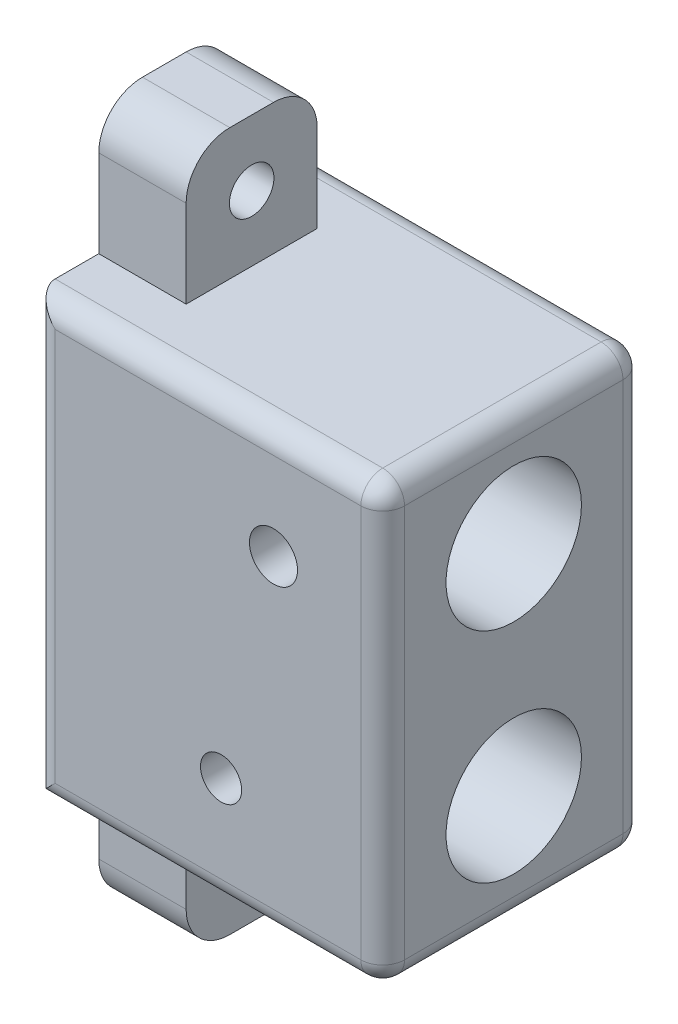
SolidWorks part; units mm, degrees
ref_plane "Front Plane" through (0, 0, 0) normal (0, 0, 1) x (1, 0, 0)
ref_plane "Top Plane" through (0, 0, 0) normal (0, 1, 0) x (1, 0, 0)
ref_plane "Right Plane" through (0, 0, 0) normal (1, 0, 0) x (0, 0, -1)
sketch "Sketch1" plane through (0, 0, 0) normal (0, 1, 0) x (1, 0, 0)
  line L0 (0, 20) -> (20, 20)
  line L2 (0, 0) -> (0, 20)
  line L4 (20, 0) -> (20, 20)
  line L5 (20, 0) -> (80, 0)
  line L6 (0, 0) -> (0, -60)
  line L7 (0, -60) -> (80, -60)
  line L8 (80, 0) -> (80, -60)
  dimension "D1" = 20
  dimension "D2" = 80
  dimension "D3" = 20
  dimension "D4" = 60
extrude "Boss-Extrude1" add sketch "Sketch1" along normal blind 100
sketch "Sketch2" plane through (80, 0, 0) normal (1, 0, 0) x (0, 0, -1)
  line L0 (0, 100) -> (0, 0) construction
  line L1 (0, 100) -> (0, 0) construction
  line L2 (-60, 0) -> (0, 0) construction
  line L3 (-60, 100) -> (0, 100) construction
  circle A0 centre (-30, 75) radius 15.5
  circle A1 centre (-30, 25) radius 15.5
  dimension "D1" = 31
  dimension "D2" = 31
  dimension "D4" = 30
  dimension "D5" = 25
  dimension "D6" = 25
  dimension "D3" = 30
extrude "Cut-Extrude1" cut sketch "Sketch2" against normal blind 70
sketch "Sketch3" plane through (20, 0, 0) normal (1, 0, 0) x (0, 0, -1)
  line L0 (20, 100) -> (20, 0) construction
  line L1 (0, 0) -> (20, 0) construction
  circle A0 centre (10, 87.5) radius 5.1
  circle A1 centre (10, 12.5) radius 5.1
  circle A2 centre (10, 50) radius 5.1
  dimension "D1" = 10
  dimension "D2" = 10
  dimension "D3" = 10.2
  dimension "D4" = 10.2
  dimension "D5" = 75
  dimension "D6" = 12.5
  dimension "D7" = 10.2
  dimension "D8" = 10
  dimension "D9" = 37.5
extrude "Cut-Extrude2" cut sketch "Sketch3" against normal blind 70
sketch "Sketch4" plane through (0, 0, 0) normal (0, 0, -1) x (-1, 0, 0)
  line L0 (-80, 100) -> (-80, 0) construction
  line L1 (-80, 0) -> (-20, 0) construction
  line L2 (-80, 100) -> (-20, 100) construction
  circle A0 centre (-55, 75) radius 5.5
  circle A1 centre (-43, 25) radius 4.7053
  dimension "D1" = 11
  dimension "D2" = 25
  dimension "D3" = 37
  dimension "D4" = 25
  dimension "D5" = 25
extrude "Cut-Extrude3" cut sketch "Sketch4" against normal blind 70
sketch "Sketch5" plane through (0, 0, 0) normal (-1, 0, 0) x (0, 0, 1)
  line L0 (60, 100) -> (60, 0) construction
  line L5 (25, 130) -> (35, 130)
  line L6 (15, 120) -> (15, -20)
  line L7 (25, -30) -> (35, -30)
  line L8 (45, 120) -> (45, -20)
  line L9 (-20, 100) -> (60, 100) construction
  line L10 (-20, 0) -> (60, 0) construction
  circle A0 centre (30, 115) radius 5.1
  circle A1 centre (30, -15) radius 5.1
  arc A2 (15, -20) -> (25, -30) centre (25, -20) ccw
  arc A3 (35, -30) -> (45, -20) centre (35, -20) ccw
  arc A4 (35, 130) -> (45, 120) centre (35, 120) cw
  arc A5 (25, 130) -> (15, 120) centre (25, 120) ccw
  point P20 (45, 130)
  point P23 (15, 130)
  dimension "D5" = 10.2
  dimension "D6" = 15
  dimension "D7" = 15
  dimension "D8" = 10.2
  dimension "D9" = 15
  dimension "D10" = 15
  dimension "D11" = 10
  dimension "D1" = 30
  dimension "D2" = 15
  dimension "D3" = 30
  dimension "D4" = 30
extrude "Boss-Extrude2" add sketch "Sketch5" against normal blind 20
sketch "Sketch6" plane through (20, 0, 0) normal (1, 0, 0) x (0, 0, -1)
  line L4 (0, 0) -> (20, 0)
  line L5 (20, 0) -> (20, 100)
  line L6 (20, 100) -> (0, 100)
  line L7 (0, 100) -> (0, 0)
  line L8 (0, 0) -> (20, 0)
  line L9 (20, 0) -> (20, 100)
  line L10 (20, 100) -> (0, 100)
  line L11 (0, 100) -> (0, 0)
  dimension "D1" = 0
extrude "Cut-Extrude4" cut sketch "Sketch6" against normal blind 20
fillet "Fillet1" radius 5 10 edges at (0, 50, 60) (0, 50, 0) (80, 0, 30) (80, 50, 60) (80, 100, 30) (80, 50, 0) (40, 0, 60) (40, 100, 60) (40, 100, 0) (40, 0, 0)
